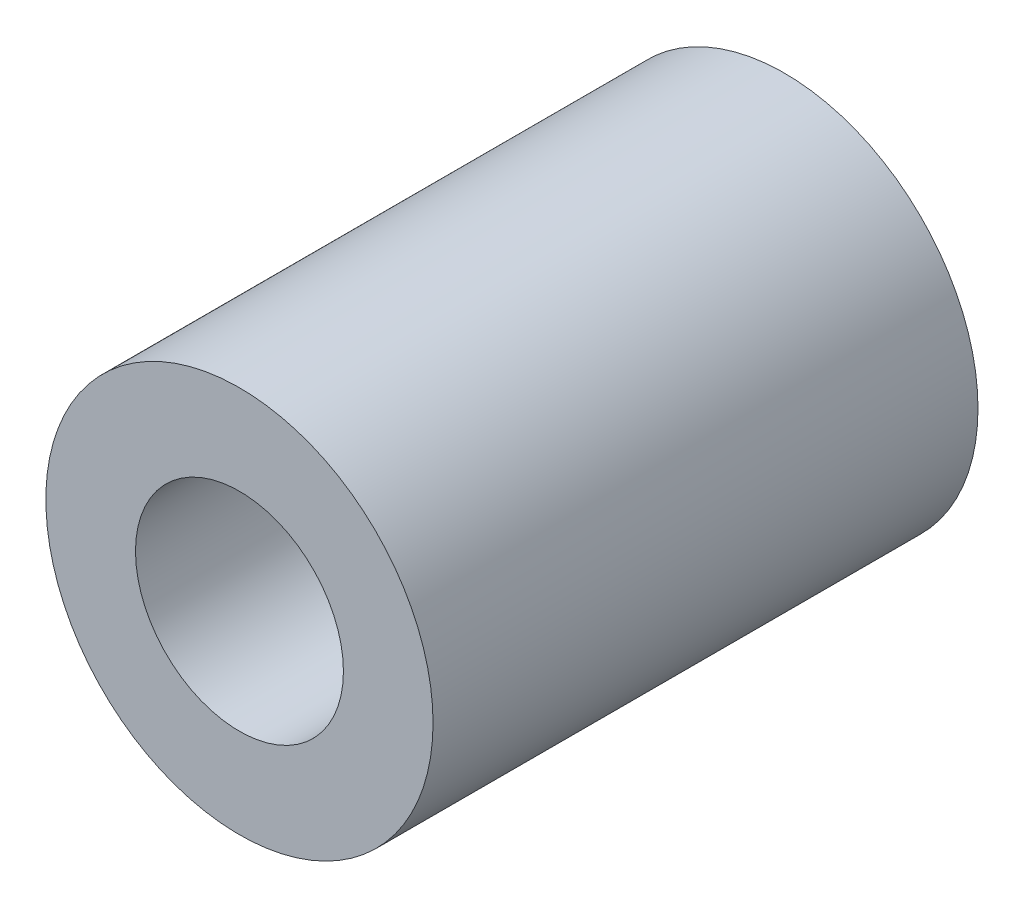
SolidWorks part; units mm, degrees
ref_plane "Front Plane" through (0, 0, 0) normal (0, 0, 1) x (1, 0, 0)
ref_plane "Top Plane" through (0, 0, 0) normal (0, 1, 0) x (1, 0, 0)
ref_plane "Right Plane" through (0, 0, 0) normal (1, 0, 0) x (0, 0, -1)
sketch "Sketch1" plane through (0, 0, 0) normal (0, 0, 1) x (1, 0, 0)
  circle A0 centre (0, 0) radius 6.5
  circle A1 centre (0, 0) radius 13.5
  dimension "D1" = 27
  dimension "D2" = 13
extrude "Boss-Extrude1" add sketch "Sketch1" along normal blind 38
hole_wizard "M16x1.5 Tapped Hole1" positions "Sketch5" profile "Sketch4" tap size "M16x1.5" standard "Iso" end condition through all
sketch "Sketch5" plane through (0, 0, 0) normal (0, 0, -1) x (-1, 0, 0)
  point P0 (0, 0)
cosmetic thread "Cosmetic Thread1" parameters "D2"=16
sketch "Sketch4" plane through (0, 0, 0) normal (1, 0, 0) x (0, 1, 0)
  line L0 (0, 0) -> (0, 38)
  line L1 (0, 38) -> (7.25, 38)
  line L2 (7.25, 38) -> (7.25, 0)
  line L5 (7.25, 0) -> (0, 0)
  line L11 (0, -6.35) -> (0, 107.95) construction
  dimension "通孔螺纹孔钻头直径" = 14.5
  dimension "通孔螺纹孔钻头深度" = 38
